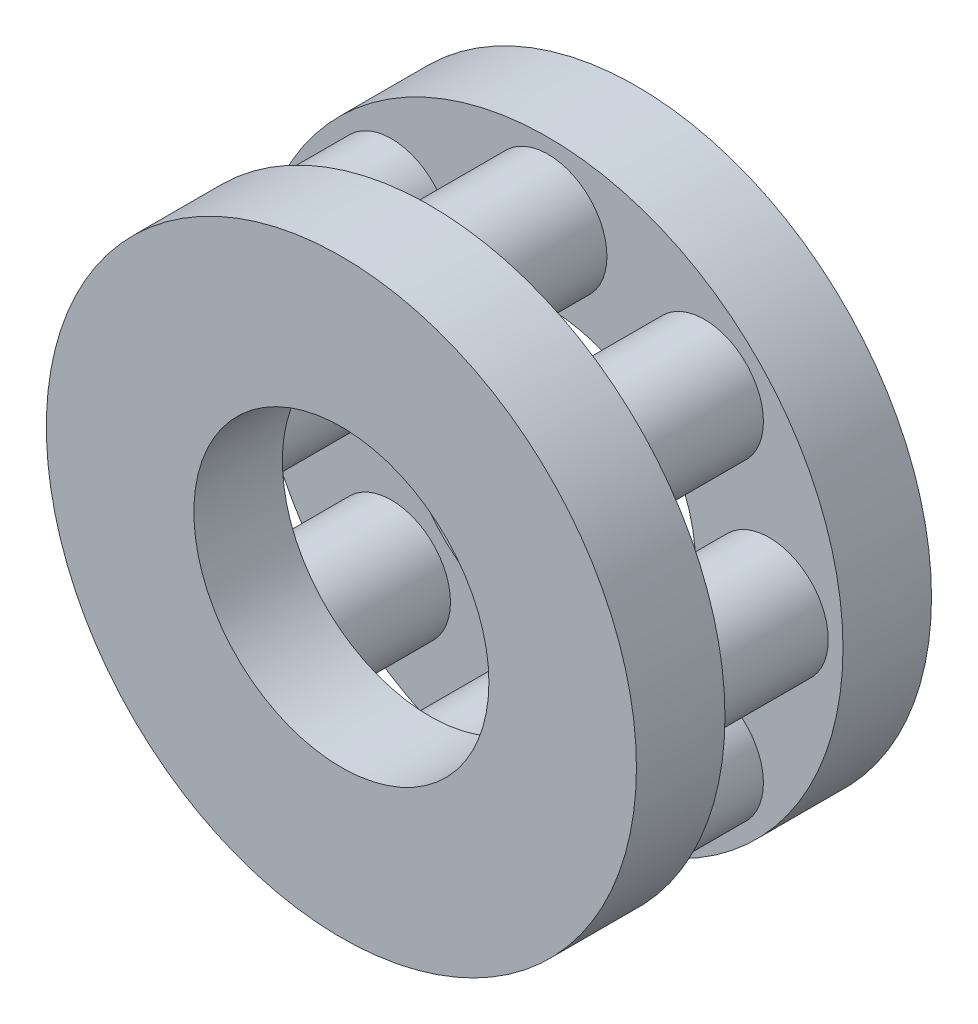
from build123d import *

# Parameters (mm, degrees)
BOSS_EXTRUDE1_START = 1
SKETCH4_4_R         = 5
SKETCH4_4_R_2       = 2.5
BOSS_EXTRUDE1_DEPTH = 1.5
BOSS_EXTRUDE2_START = -1
SKETCH_4_4_R        = 5
SKETCH_4_4_R_2      = 2.5
BOSS_EXTRUDE2_DEPTH = 1.5
SKETCH8_R           = 1
BOSS_EXTRUDE3_DEPTH = 2


with BuildPart() as part:
    # Sketch4<4> → Boss-Extrude1 (new body)
    with BuildSketch(Plane.XY.offset(BOSS_EXTRUDE1_START)):
        Circle(SKETCH4_4_R)
        Circle(SKETCH4_4_R_2, mode=Mode.SUBTRACT)
    extrude(amount=BOSS_EXTRUDE1_DEPTH)



with BuildPart() as body_2:
    # 草图4<4> → Boss-Extrude2 (new body)
    with BuildSketch(Plane.XY.offset(BOSS_EXTRUDE2_START)):
        Circle(SKETCH_4_4_R)
        Circle(SKETCH_4_4_R_2, mode=Mode.SUBTRACT)
    extrude(amount=-BOSS_EXTRUDE2_DEPTH)


with BuildPart() as part_1:
    add(part.part)

    add(body_2.part)  # Boss-Extrude3 merges body 2
    # Sketch8 → Boss-Extrude3 (add)
    with BuildSketch(Plane.XY.offset(-1)):
        with Locations((0, 3.75)):
            Circle(SKETCH8_R)
        with Locations((2.651650429, 2.651650429)):
            Circle(SKETCH8_R)
        with Locations((3.75, 0)):
            Circle(SKETCH8_R)
        with Locations((2.651650429, -2.651650429)):
            Circle(SKETCH8_R)
        with Locations((0, -3.75)):
            Circle(SKETCH8_R)
        with Locations((-2.651650429, -2.651650429)):
            Circle(SKETCH8_R)
        with Locations((-3.75, 0)):
            Circle(SKETCH8_R)
        with Locations((-2.651650429, 2.651650429)):
            Circle(SKETCH8_R)
    extrude(amount=BOSS_EXTRUDE3_DEPTH)


solid = part_1.part
